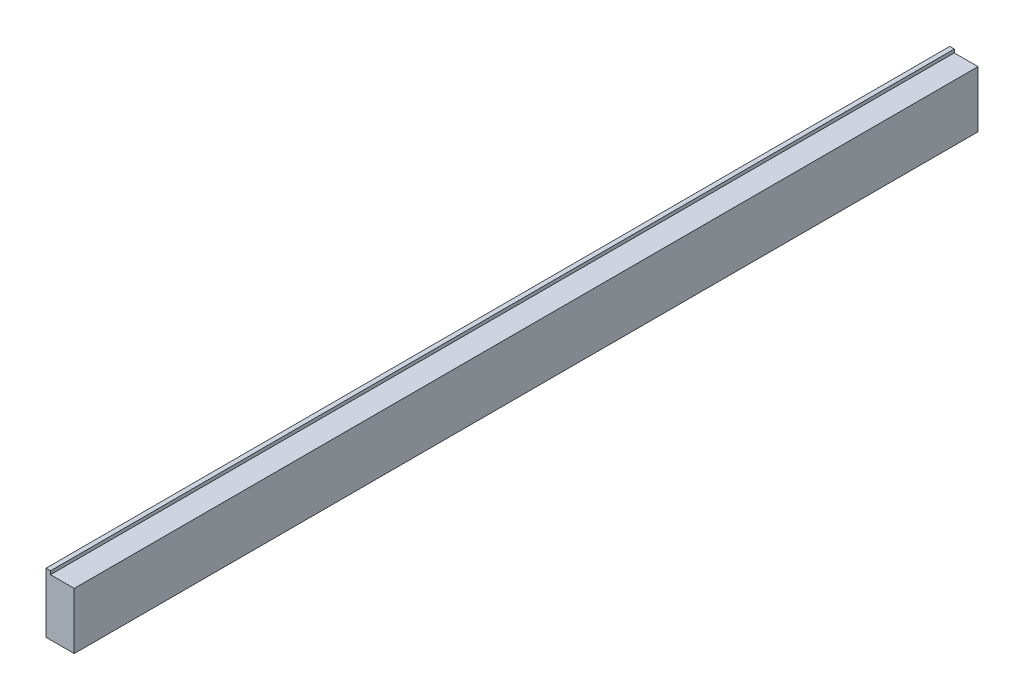
SolidWorks part; units mm, degrees
ref_plane "前视基准面" through (0, 0, 0) normal (0, 0, 1) x (1, 0, 0)
ref_plane "上视基准面" through (0, 0, 0) normal (0, 1, 0) x (1, 0, 0)
ref_plane "右视基准面" through (0, 0, 0) normal (1, 0, 0) x (0, 0, -1)
sketch "草图1" plane through (0, 0, 0) normal (0, 0, 1) x (1, 0, 0)
  line L0 (-10, -12.5) -> (-14, -12.5)
  line L1 (-10, -10.2831) -> (-10, -14.5) construction
  line L2 (-14, -12.5) -> (-14, -65.5)
  line L3 (-14, -65.5) -> (11, -65.5)
  line L4 (11, -65.5) -> (11, -15.5)
  line L5 (11, -15.5) -> (-10, -15.5)
  line L6 (-10, -15.5) -> (-10, -12.5)
  dimension "D1" = 50
  dimension "D2" = 3
  dimension "D3" = 4
  dimension "D4" = 25
  dimension "D5" = 15.5
extrude "凸台-拉伸1" add sketch "草图1" against normal up to surface (800 mm away)
